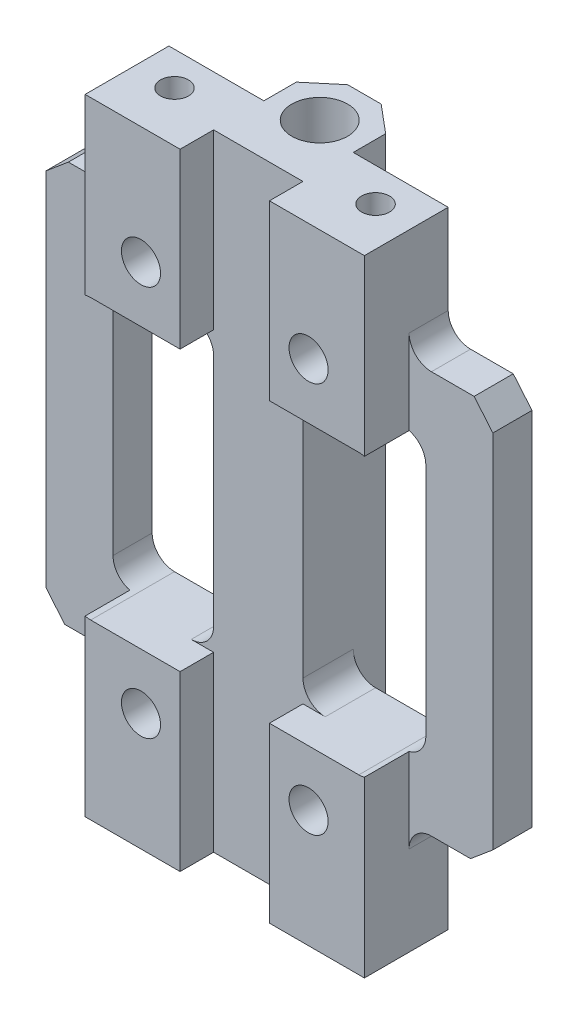
SolidWorks part; units mm, degrees
material "AISI 304"
ref_plane "Front Plane" through (0, 0, 0) normal (0, 0, 1) x (1, 0, 0)
ref_plane "Top Plane" through (0, 0, 0) normal (0, 1, 0) x (1, 0, 0)
ref_plane "Right Plane" through (0, 0, 0) normal (1, 0, 0) x (0, 0, -1)
sketch "Sketch1" plane through (0, 0, 0) normal (0, 1, 0) x (1, 0, 0)
  line L0 (0, 0) -> (0, -50000) construction
  line L1 (-12.5, 6.25) -> (12.5, 6.25)
  line L2 (-12.5, 6.25) -> (-12.5, -6.25)
  line L3 (-12.5, -6.25) -> (12.5, -6.25)
  line L4 (12.5, 6.25) -> (12.5, -6.25)
  line L5 (-12.5, 6.25) -> (12.5, -6.25) construction
  line L6 (-12.5, -6.25) -> (12.5, 6.25) construction
  line L12 (-2.45, -5) -> (2.45, -1) construction
  line L13 (-2.45, -1) -> (2.45, -5) construction
  line L18 (-2.5289, -24.1834) -> (2.05, -2.5) construction
  line L19 (-2.05, -2.5) -> (2.8719, -25.8076) construction
  point P0 (0, 0)
  point P8 (0, -3)
  point P13 (0, -12.2077)
  dimension "D1" = 25
  dimension "D2" = 12.5
extrude "Boss-Extrude1" add sketch "Sketch1" along normal blind 56
sketch "Sketch3" plane through (0, 0, -6.25) normal (0, 0, -1) x (-1, 0, 0)
  line L0 (0, 0) -> (0, 50000) construction
  line L1 (-12.5, 0) -> (12.5, 0) construction
  line L2 (-12.5, 56) -> (-4, 56)
  line L3 (-12.5, 56) -> (-12.5, 0)
  line L4 (-12.5, 0) -> (-4, 0)
  line L5 (-4, 56) -> (-4, 0)
  line L6 (12.5, 0) -> (4, 0)
  line L7 (4, 56) -> (4, 0)
  line L8 (12.5, 56) -> (4, 56)
  line L9 (12.5, 56) -> (12.5, 0)
  dimension "D1" = 8
extrude "Cut-Extrude2" cut sketch "Sketch3" against normal blind 5
sketch "Sketch4" plane through (0, 0, 0) normal (0, -1, 0) x (1, 0, 0)
  line L0 (0, 0) -> (0, -50000) construction
  line L1 (4, -6.25) -> (-4, -6.25) construction
  circle A0 centre (0, -2.25) radius 2.5
  dimension "D1" = 5
  dimension "D2" = 4
extrude "Cut-Extrude3" cut sketch "Sketch4" against normal through all
sketch "Sketch5" plane through (0, 0, -1.25) normal (0, 0, -1) x (-1, 0, 0)
  line L0 (0, 46) -> (0, -49954) construction
  line L1 (-4, 56) -> (4, 56) construction
  line L2 (-12.5, 28) -> (49987.5, 28) construction
  line L3 (-12.5, 56) -> (-12.5, 0) construction
  circle A0 centre (-7.5, 45.5) radius 1.75
  circle A1 centre (7.5, 45.5) radius 1.75
  circle A2 centre (7.5, 10.5) radius 1.75
  circle A3 centre (-7.5, 10.5) radius 1.75
  point P4 (0, 56)
  point P9 (-12.5, 28)
  dimension "D3" = 3.5
  dimension "D1" = 35
  dimension "D2" = 15
extrude "Cut-Extrude4" cut sketch "Sketch5" against normal through all
sketch "Sketch6" plane through (0, 0, -1.25) normal (0, 0, -1) x (-1, 0, 0)
  circle A0 centre (-7.5, 45.5) radius 3
  circle A1 centre (7.5, 45.5) radius 3
  circle A2 centre (7.5, 10.5) radius 3
  circle A3 centre (-7.5, 10.5) radius 3
  dimension "D1" = 6
extrude "Cut-Extrude5" cut sketch "Sketch6" against normal blind 3.5
chamfer "Chamfer1" distance 2.5 angle 40 2 edges at (-4, 28, -6.25) (4, 28, -6.25)
sketch "Sketch8" plane through (0, 0, -1.25) normal (0, 0, -1) x (-1, 0, 0)
  line L0 (0, 56) -> (0, -49944) construction
  line L1 (-1.5, 56) -> (1.5, 56) construction
  line L2 (12.5, 28) -> (-49987.5, 28) construction
  line L3 (12.5, 0) -> (12.5, 56) construction
  line L4 (-12.5, 56) -> (-12.5, 0) construction
  line L5 (-12.5, 46) -> (-20, 46)
  line L6 (-12.5, 46) -> (-12.5, 10)
  line L7 (-12.5, 10) -> (-20, 10)
  line L8 (-20, 46) -> (-20, 10)
  line L9 (20, 46) -> (20, 10)
  line L10 (12.5, 10) -> (20, 10)
  line L11 (12.5, 46) -> (12.5, 10)
  line L12 (12.5, 46) -> (20, 46)
  point P4 (0, 56)
  point P9 (12.5, 28)
  dimension "D1" = 36
  dimension "D2" = 7.5
extrude "Boss-Extrude3" add sketch "Sketch8" against normal blind 3.5
hole_wizard "M3 Tapped Hole1" positions "Sketch10" profile "Sketch9" tap size "M3" standard "Gb"
sketch "Sketch10" plane through (0, 0, 0) normal (0, -1, 0) x (-1, 0, 0)
  point P0 (-9, -1.75)
  point P3 (9, -1.75)
sketch "Sketch9" plane through (9, 0, 1.75) normal (1, 0, 0) x (0, 0, -1)
  line L0 (0, 0) -> (0, 8.2511)
  line L1 (0, 8.2511) -> (1.25, 7.5)
  line L2 (1.25, 7.5) -> (1.25, 0)
  line L5 (1.25, 0) -> (0, 0)
  line L10 (0, 8.2511) -> (-1.25, 7.5) construction
  line L11 (0, -6.35) -> (0, 107.95) construction
  dimension "螺纹孔钻头直径" = 2.5
  dimension "螺纹孔钻头深度" = 7.5
  dimension "导头角度" = 118
cosmetic thread "Cosmetic thread 5" parameters "D1"=6, "D2"=3
cosmetic thread "Cosmetic thread 6" parameters "D1"=6, "D2"=3
hole_wizard "M3 Tapped Hole2" positions "Sketch12" profile "Sketch11" tap size "M3" standard "Gb"
sketch "Sketch12" plane through (0, 56, 0) normal (0, 1, 0) x (1, 0, 0)
  point P0 (-9, -1.75)
  point P3 (9, -1.75)
sketch "Sketch11" plane through (-9, 56, 1.75) normal (1, 0, 0) x (0, 0, 1)
  line L0 (0, 0) -> (0, 8.2511)
  line L1 (0, 8.2511) -> (1.25, 7.5)
  line L2 (1.25, 7.5) -> (1.25, 0)
  line L5 (1.25, 0) -> (0, 0)
  line L10 (0, 8.2511) -> (-1.25, 7.5) construction
  line L11 (0, -6.35) -> (0, 107.95) construction
  dimension "螺纹孔钻头直径" = 2.5
  dimension "螺纹孔钻头深度" = 7.5
  dimension "导头角度" = 118
cosmetic thread "Cosmetic thread 7" parameters "D1"=6, "D2"=3
cosmetic thread "Cosmetic thread 8" parameters "D1"=6, "D2"=3
chamfer "Chamfer2" distance 2 angle 40 4 edges at (-20, 46, 0.5) (20, 46, 0.5) (20, 10, 0.5) (-20, 10, 0.5)
fillet "Fillet1" radius 2 4 edges
sketch "Sketch16" plane through (0, 0, 6.25) normal (0, 0, 1) x (1, 0, 0)
  line L0 (-12.5, 0) -> (12.5, 0) construction
  line L2 (0, 56) -> (0, -49944) construction
  line L3 (-12.5, 56) -> (12.5, 56) construction
  line L4 (4, 40.5) -> (8.5, 40.5)
  line L5 (-8.5, 15.5) -> (-4, 15.5)
  line L6 (-8.5, 15.5) -> (-8.5, 40.5)
  line L7 (-8.5, 40.5) -> (-4, 40.5)
  line L8 (8.5, 15.5) -> (8.5, 40.5)
  line L9 (-8.5, 15.5) -> (8.5, 40.5) construction
  line L10 (-8.5, 40.5) -> (8.5, 15.5) construction
  line L11 (-4, 56) -> (4, 56)
  line L12 (-4, 56) -> (-4, 40.5)
  line L13 (-4, 0) -> (4, 0)
  line L14 (4, 56) -> (4, 40.5)
  line L15 (-4, 56) -> (4, 40.5) construction
  line L16 (-4, 40.5) -> (4, 56) construction
  line L17 (-4, 0) -> (-4, 15.5)
  line L18 (4, 0) -> (4, 15.5)
  line L19 (4, 15.5) -> (8.5, 15.5)
  line L20 (-8.5, 28) -> (49991.5, 28) construction
  point P4 (-8.5, 28)
  point P9 (0, 56)
  point P10 (0, 28)
  point P15 (0, 48.25)
  dimension "D1" = 17
  dimension "D2" = 25
  dimension "D3" = 8
extrude "Cut-Extrude7" cut sketch "Sketch16" against normal blind 3
sketch "Sketch17" plane through (0, 0, -1.25) normal (0, 0, -1) x (-1, 0, 0)
  line L0 (-20, 28) -> (49980, 28) construction
  line L1 (-20, 44) -> (-20, 11.6782) construction
  line L2 (0, 56) -> (0, -49944) construction
  line L3 (-1.5, 56) -> (1.5, 56) construction
  line L4 (-4, 0) -> (-4, 56) construction
  line L5 (-14, 40.5) -> (-4, 40.5)
  line L6 (14, 40.5) -> (14, 15.5)
  line L7 (-14, 15.5) -> (-4, 15.5)
  line L8 (-4, 40.5) -> (-4, 15.5)
  line L9 (-35.3857, 39.7044) -> (-4, 15.5) construction
  line L10 (-34.5156, 16.3528) -> (-4, 40.5) construction
  line L11 (34.5156, 16.3528) -> (4, 40.5) construction
  line L12 (35.3857, 39.7044) -> (4, 15.5) construction
  line L13 (4, 40.5) -> (4, 15.5)
  line L14 (14, 15.5) -> (4, 15.5)
  line L15 (-14, 40.5) -> (-14, 15.5)
  line L16 (14, 40.5) -> (4, 40.5)
  line L17 (12.5, 56) -> (4, 56) construction
  line L18 (4, 0) -> (12.5, 0) construction
  point P9 (0, 56)
  point P10 (-20, 27.8391)
  point P21 (20, 27.8391)
  dimension "D1" = 10
  dimension "D2" = 25
extrude "Cut-Extrude8" cut sketch "Sketch17" against normal blind 10
fillet "Fillet3" radius 2 8 edges at (-4, 15.5, 1) (4, 15.5, 1) (4, 40.5, 1) (-14, 40.5, 0.5) (-14, 15.5, 0.5) (14, 15.5, 0.5) (14, 40.5, 0.5) (-4, 40.5, 1)
